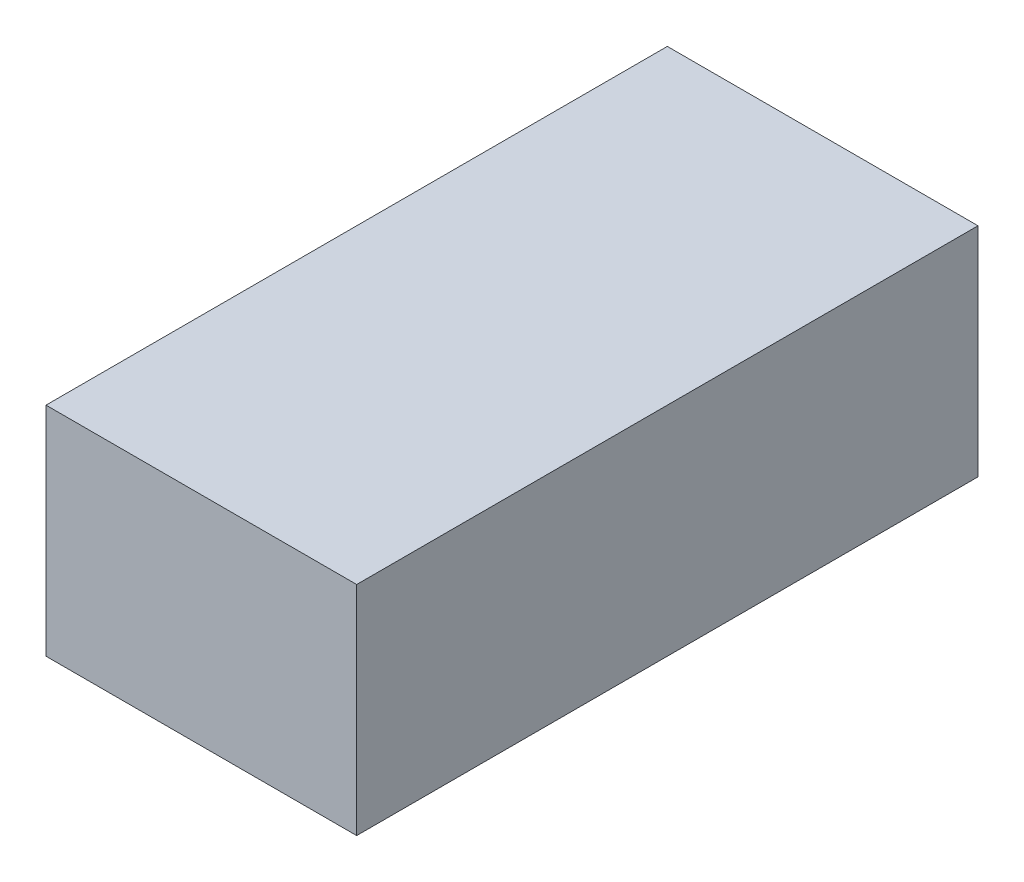
from build123d import *

# Parameters (mm, degrees)
SKETCH_1_W      = 300
SKETCH_1_H      = 210
EXTRUDE_1_DEPTH = 600


with BuildPart() as part:
    # 草图1 → 凸台-拉伸1 (new body)
    with BuildSketch(Plane.XY):
        Rectangle(SKETCH_1_W, SKETCH_1_H)
    extrude(amount=EXTRUDE_1_DEPTH)


solid = part.part
